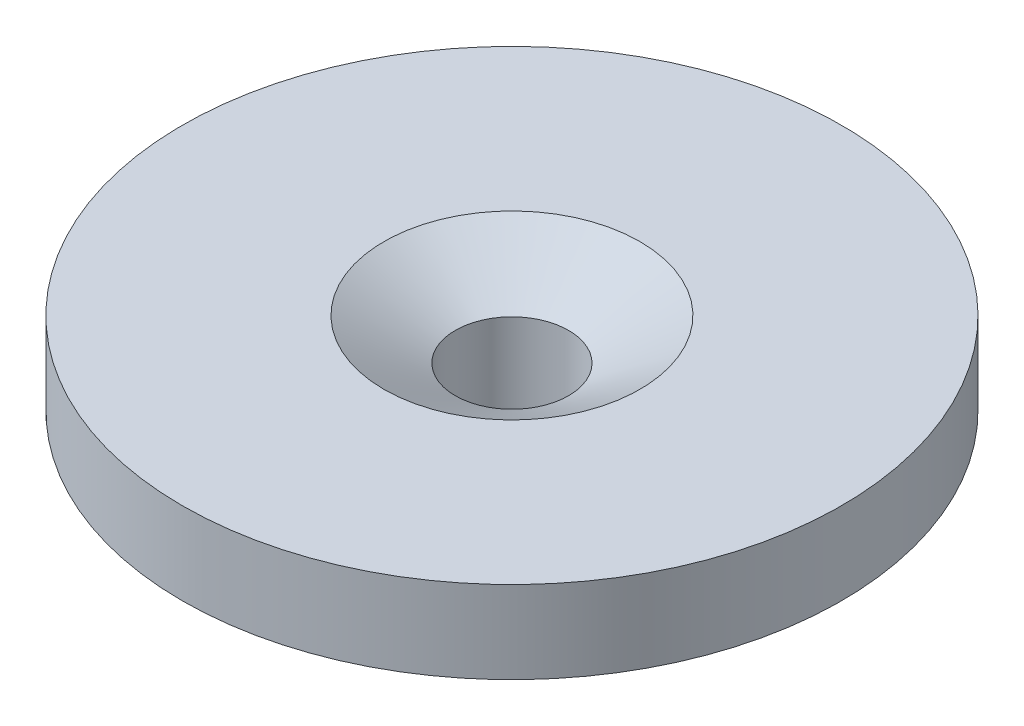
from build123d import *


with BuildPart() as part:
    # Sketch1 → Revolve1 (revolve)
    with BuildSketch(Plane.XY, mode=Mode.PRIVATE) as revolve1_sk:
        Polygon((-2.75, -2.226189364), (-9, -2.226189364), (-9, 1.773810636), (-14, 1.773810636), (-14, -0.226189364), (-16, -0.226189364), (-16, 3.773810636), (-6.214101615, 3.773810636), (-2.75, 1.773810636), align=None)
    revolve(revolve1_sk.sketch.rotate(Axis((0, 9.90888507, 0), (0, -1, 0)), 270), axis=Axis((0, 9.90888507, 0), (0, -1, 0)))


solid = part.part
